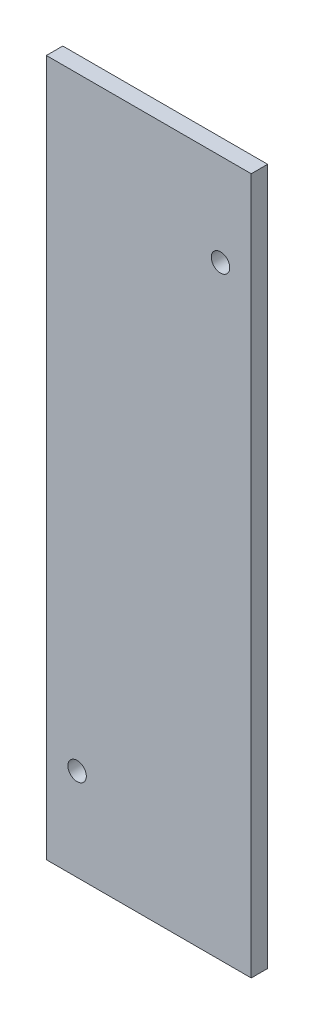
SolidWorks part; units mm, degrees
ref_plane "前视基准面" through (0, 0, 0) normal (0, 0, 1) x (1, 0, 0)
ref_plane "上视基准面" through (0, 0, 0) normal (0, 1, 0) x (1, 0, 0)
ref_plane "右视基准面" through (0, 0, 0) normal (1, 0, 0) x (0, 0, -1)
other "Configuration Table"
sketch "草图1" plane through (0, 0, 0) normal (0, 0, 1) x (1, 0, 0)
  line L0 (-50, -170) -> (50, -170)
  line L1 (50, -170) -> (50, 170)
  line L2 (50, 170) -> (-50, 170)
  line L3 (-50, 170) -> (-50, -170)
  point P0 (0, 0)
  dimension "D1" = 50
  dimension "D2" = 100
  dimension "D3" = 170
  dimension "D4" = 340
extrude "凸台-拉伸1" add sketch "草图1" against normal mid plane 8
sketch "草图2" plane through (0, 0, 0) normal (0, 0, 1) x (1, 0, 0)
  circle A0 centre (-35, -125) radius 4.5
  circle A1 centre (35, 125) radius 4.5
  point P0 (0, 0)
  dimension "D1" = 9
  dimension "D2" = 9
  dimension "D3" = 35
  dimension "D4" = 70
  dimension "D5" = 125
  dimension "D6" = 250
extrude "切除-拉伸1" cut sketch "草图2" against normal mid plane 28
